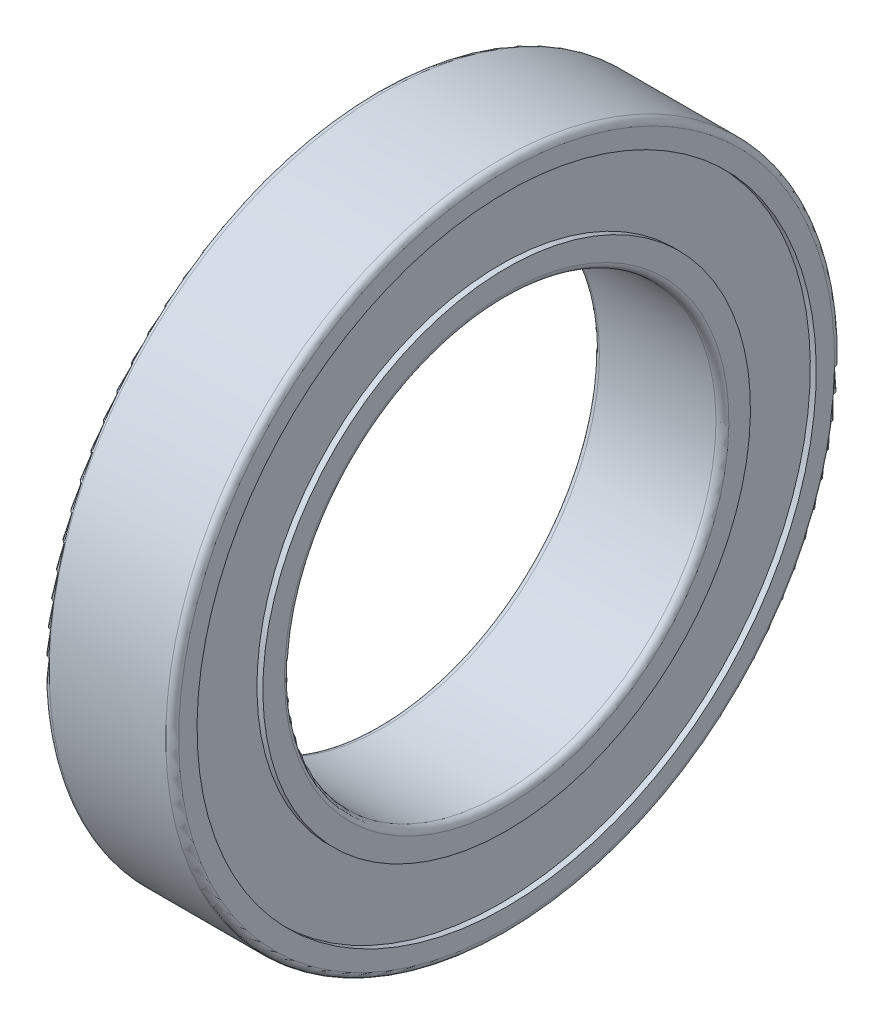
from build123d import *

# Parameters (mm, degrees)
FILLET1_R = 0.6
FILLET2_R = 0.6


with BuildPart() as part:
    # Sketch1 → Revolve1 (revolve)
    with BuildSketch(Plane.XY, mode=Mode.PRIVATE) as revolve1_sk:
        Polygon((0, 20), (12, 20), (12, 22.6), (11.45, 22.6), (11.45, 28.7), (12, 28.7), (12, 31), (0, 31), (0, 28.7), (0.55, 28.7), (0.55, 22.6), (0, 22.6), align=None)
    revolve(revolve1_sk.sketch.rotate(Axis((0, 0, 0), (1, 0, 0)), 180), axis=Axis((0, 0, 0), (1, 0, 0)))

    # Fillet1
    fillet1_edges = [part.edges().sort_by_distance(p)[0] for p in [
        (0, 31, 0),
        (12, 31, 0),
    ]]
    fillet(fillet1_edges, radius=FILLET1_R)

    # Fillet2
    fillet2_edges = [part.edges().sort_by_distance(p)[0] for p in [
        (12, 20, 0),
        (0, 20, 0),
    ]]
    fillet(fillet2_edges, radius=FILLET2_R)


solid = part.part
